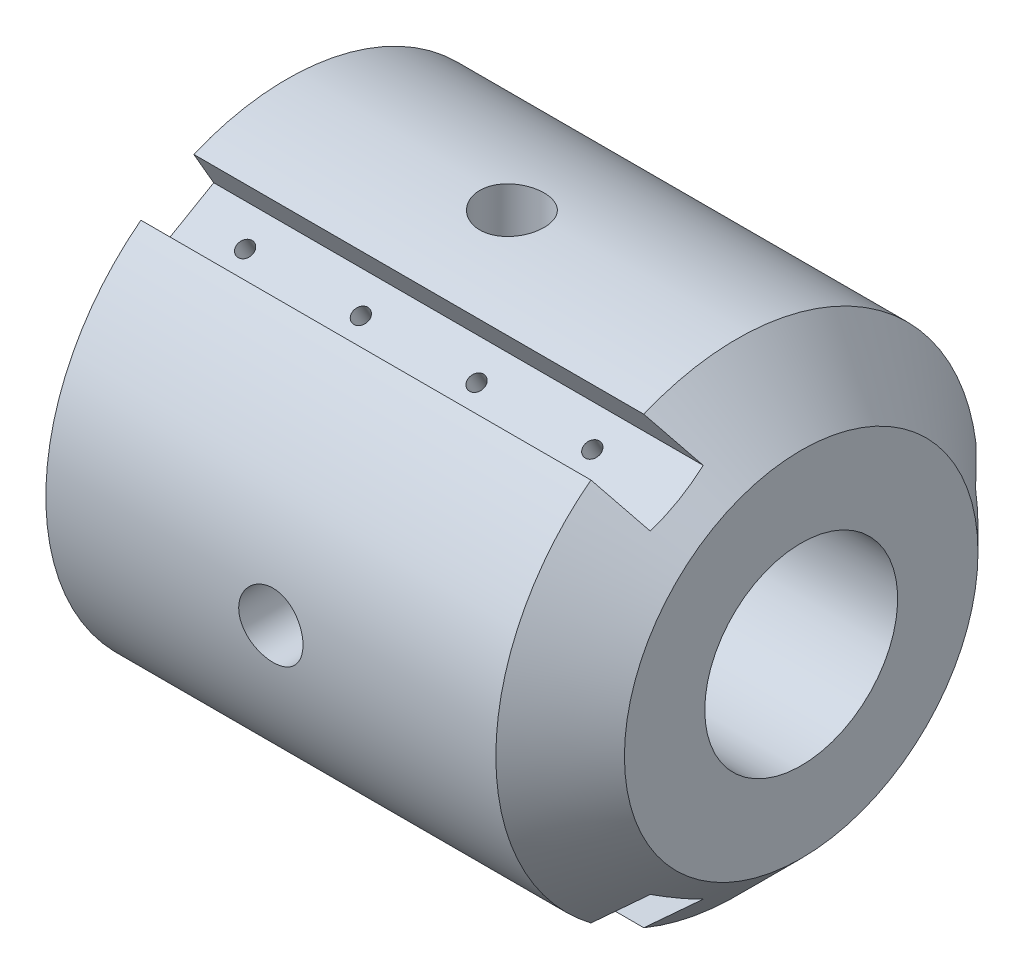
from build123d import *

# Parameters (mm, degrees)
SKETCH1_W                  = 80
SKETCH1_H                  = 22.5
CHAMFER1_SIZE              = 10
CUT_EXTRUDE1_START         = 22.5
SKETCH2_R                  = 5
CUT_EXTRUDE1_DEPTH         = 74.481769102
CIRPATTERN1_COUNT          = 2
CIRPATTERN1_ANGLE          = 90
SKETCH5_W                  = 13
SKETCH5_H                  = 9.5
CUT_EXTRUDE2_DEPTH         = 96.981769264
M3_TAPPED_HOLE1_AT_2_COUNT = 2
M3_TAPPED_HOLE1_AT_2_PITCH = 18
M3_TAPPED_HOLE1_AT_3_COUNT = 2
M3_TAPPED_HOLE1_AT_3_PITCH = 18
M3_TAPPED_HOLE1_AT_4_COUNT = 2
M3_TAPPED_HOLE1_AT_4_PITCH = 36
CIRPATTERN2_COUNT          = 3


with BuildPart() as part:
    # Sketch1 → Revolve1 (revolve)
    with BuildSketch(Plane.XY, mode=Mode.PRIVATE) as revolve1_sk:
        with Locations((40, 26.25)):
            Rectangle(SKETCH1_W, SKETCH1_H)
    revolve(revolve1_sk.sketch.rotate(Axis((0, 0, 0), (1, 0, 0)), 90), axis=Axis((0, 0, 0), (1, 0, 0)))

    # Chamfer1
    chamfer1_edges = [part.edges().sort_by_distance(p)[0] for p in [
        (80, 0, -37.5),
    ]]
    chamfer(chamfer1_edges, length=CHAMFER1_SIZE)

    # Sketch2 → Cut-Extrude1 (cut, through all)
    with BuildSketch(Plane.XY.offset(CUT_EXTRUDE1_START)):
        with Locations((35, 0)):
            Circle(SKETCH2_R)
    cut_extrude1 = extrude(amount=CUT_EXTRUDE1_DEPTH, mode=Mode.SUBTRACT)

    # Sketch3 → M5 Tapped Hole1 (revolve, cut)
    with BuildSketch(Plane(origin=(35, 0, 22.5), x_dir=(0, -1, 0), z_dir=(1, 0, 0))):
        Polygon((0, 0), (0, 13.6618073), (2.1, 12.4), (2.1, 0), align=None)
    m5_tapped_hole1 = revolve(axis=Axis((35, 0, 28.85), (0, 0, -1)), mode=Mode.SUBTRACT)

    # CirPattern1: Cut-Extrude1, M5 Tapped Hole1 ×2 about axis
    cirpattern1_axis = Axis((0, 0, 0), (-1, 0, 0))
    add([cut_extrude1.rotate(cirpattern1_axis, i * CIRPATTERN1_ANGLE / (CIRPATTERN1_COUNT - 1)) for i in range(1, CIRPATTERN1_COUNT)], mode=Mode.SUBTRACT)
    add([m5_tapped_hole1.rotate(cirpattern1_axis, i * CIRPATTERN1_ANGLE / (CIRPATTERN1_COUNT - 1)) for i in range(1, CIRPATTERN1_COUNT)], mode=Mode.SUBTRACT)

    # Sketch5 → Cut-Extrude2 (cut, through all)
    with BuildSketch(Plane(origin=(80, 0, 0), x_dir=(0, 0, -1), z_dir=(1, 0, 0))):
        with Locations((37.5, 0)):
            Rectangle(SKETCH5_W, SKETCH5_H)
    cut_extrude2 = extrude(amount=-CUT_EXTRUDE2_DEPTH, mode=Mode.SUBTRACT)

    # Sketch6 → M3 Tapped Hole1 (revolve, cut)
    with BuildSketch(Plane(origin=(45, 0, -31), x_dir=(0, 1, 0), z_dir=(1, 0, 0))):
        Polygon((0, 0), (0, 8.251075774), (1.25, 7.5), (1.25, 0), align=None)
    m3_tapped_hole1 = revolve(axis=Axis((45, 0, -37.35), (0, 0, 1)), mode=Mode.SUBTRACT)

    # M3 Tapped Hole1 at 2: M3 Tapped Hole1 ×2
    with Locations(*[(i * M3_TAPPED_HOLE1_AT_2_PITCH, 0, 0) for i in range(1, M3_TAPPED_HOLE1_AT_2_COUNT)]):
        add(m3_tapped_hole1, mode=Mode.SUBTRACT)

    # M3 Tapped Hole1 at 3: M3 Tapped Hole1 ×2
    with Locations(*[(-i * M3_TAPPED_HOLE1_AT_3_PITCH, 0, 0) for i in range(1, M3_TAPPED_HOLE1_AT_3_COUNT)]):
        add(m3_tapped_hole1, mode=Mode.SUBTRACT)

    # M3 Tapped Hole1 at 4: M3 Tapped Hole1 ×2
    with Locations(*[(-i * M3_TAPPED_HOLE1_AT_4_PITCH, 0, 0) for i in range(1, M3_TAPPED_HOLE1_AT_4_COUNT)]):
        add(m3_tapped_hole1, mode=Mode.SUBTRACT)

    # CirPattern2: Cut-Extrude2, M3 Tapped Hole1 ×3 about axis
    cirpattern2_axis = Axis((0, 0, 0), (1, 0, 0))
    add([cut_extrude2.rotate(cirpattern2_axis, i * 360 / CIRPATTERN2_COUNT) for i in range(1, CIRPATTERN2_COUNT)], mode=Mode.SUBTRACT)
    add([m3_tapped_hole1.rotate(cirpattern2_axis, i * 360 / CIRPATTERN2_COUNT) for i in range(1, CIRPATTERN2_COUNT)], mode=Mode.SUBTRACT)

    # CirPattern2 copy 1 sketch → CirPattern2 copy 1 (revolve, cut)
    with BuildSketch(Plane(origin=(63, 26.846787517, 15.5), x_dir=(0, -0.4999999999999998, 0.8660254037844387), z_dir=(1, 0, 0))):
        Polygon((0, 0), (0, 8.251075774), (1.25, 7.5), (1.25, 0), align=None)
    revolve(axis=Axis((63, 32.346048831, 18.675), (0, -0.8660254037844387, -0.4999999999999998)), mode=Mode.SUBTRACT)

    # CirPattern2 copy 2 sketch → CirPattern2 copy 2 (revolve, cut)
    with BuildSketch(Plane(origin=(63, -26.846787517, 15.5), x_dir=(0, -0.5000000000000004, -0.8660254037844384), z_dir=(1, 0, 0))):
        Polygon((0, 0), (0, 8.251075774), (1.25, 7.5), (1.25, 0), align=None)
    revolve(axis=Axis((63, -32.346048831, 18.675), (0, 0.8660254037844384, -0.5000000000000004)), mode=Mode.SUBTRACT)

    # CirPattern2 copy 3 sketch → CirPattern2 copy 3 (revolve, cut)
    with BuildSketch(Plane(origin=(27, 26.846787517, 15.5), x_dir=(0, -0.4999999999999998, 0.8660254037844387), z_dir=(1, 0, 0))):
        Polygon((0, 0), (0, 8.251075774), (1.25, 7.5), (1.25, 0), align=None)
    revolve(axis=Axis((27, 32.346048831, 18.675), (0, -0.8660254037844387, -0.4999999999999998)), mode=Mode.SUBTRACT)

    # CirPattern2 copy 4 sketch → CirPattern2 copy 4 (revolve, cut)
    with BuildSketch(Plane(origin=(27, -26.846787517, 15.5), x_dir=(0, -0.5000000000000004, -0.8660254037844384), z_dir=(1, 0, 0))):
        Polygon((0, 0), (0, 8.251075774), (1.25, 7.5), (1.25, 0), align=None)
    revolve(axis=Axis((27, -32.346048831, 18.675), (0, 0.8660254037844384, -0.5000000000000004)), mode=Mode.SUBTRACT)

    # CirPattern2 copy 5 sketch → CirPattern2 copy 5 (revolve, cut)
    with BuildSketch(Plane(origin=(9, 26.846787517, 15.5), x_dir=(0, -0.4999999999999998, 0.8660254037844387), z_dir=(1, 0, 0))):
        Polygon((0, 0), (0, 8.251075774), (1.25, 7.5), (1.25, 0), align=None)
    revolve(axis=Axis((9, 32.346048831, 18.675), (0, -0.8660254037844387, -0.4999999999999998)), mode=Mode.SUBTRACT)

    # CirPattern2 copy 6 sketch → CirPattern2 copy 6 (revolve, cut)
    with BuildSketch(Plane(origin=(9, -26.846787517, 15.5), x_dir=(0, -0.5000000000000004, -0.8660254037844384), z_dir=(1, 0, 0))):
        Polygon((0, 0), (0, 8.251075774), (1.25, 7.5), (1.25, 0), align=None)
    revolve(axis=Axis((9, -32.346048831, 18.675), (0, 0.8660254037844384, -0.5000000000000004)), mode=Mode.SUBTRACT)


solid = part.part
